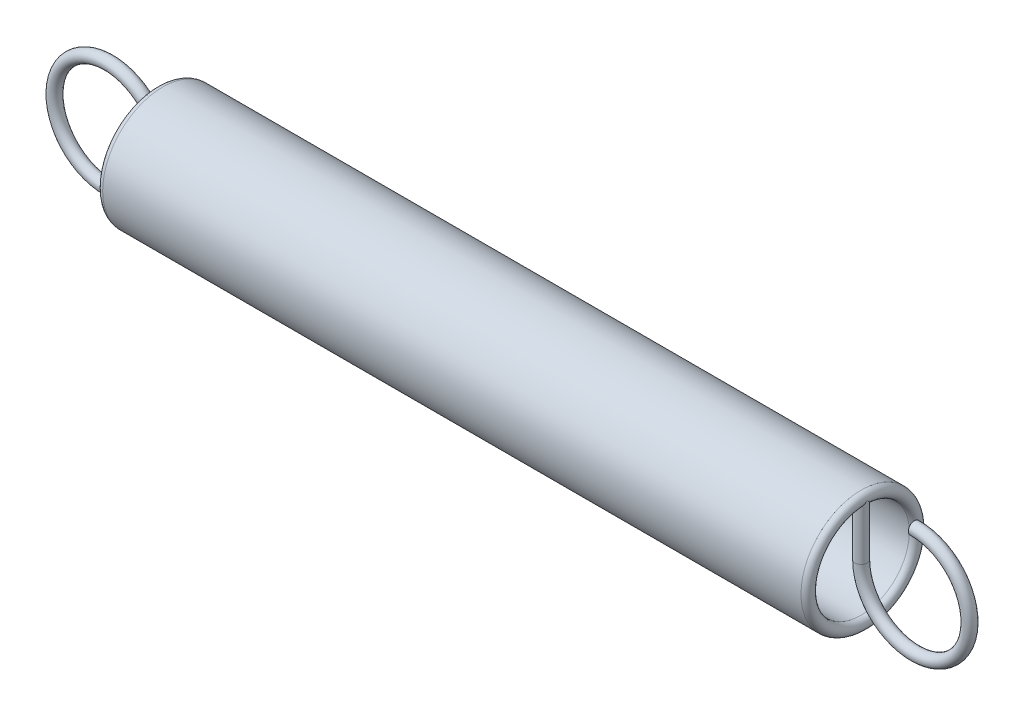
from build123d import *

# Parameters (mm, degrees)
SKETCH2_W      = 0.2
SKETCH2_H      = 1.8
SKETCH3_R      = 0.2
REVOLVE3_ANGLE = 271
SKETCH4_W      = 0.2
SKETCH4_H      = 1.8
SKETCH5_R      = 0.2
REVOLVE5_ANGLE = 271


with BuildPart() as part:
    # Sketch1 → Revolve1 (revolve)
    with BuildSketch(Plane.XY, mode=Mode.PRIVATE) as revolve1_sk:
        with BuildLine():
            Line((3.4, 1.6), (26.6, 1.6))
            ThreePointArc((26.6, 1.6), (26.8, 1.8), (26.6, 2))
            Line((26.6, 2), (3.4, 2))
            ThreePointArc((3.4, 2), (3.2, 1.8), (3.4, 1.6))
        make_face()
    revolve(revolve1_sk.sketch.rotate(Axis((26.8, 0, 0), (-1, 0, 0)), 270), axis=Axis((26.8, 0, 0), (-1, 0, 0)))

    # Sketch2 → Revolve2 (revolve)
    with BuildSketch(Plane.XY, mode=Mode.PRIVATE) as revolve2_sk:
        with Locations((26.7, 0.9)):
            Rectangle(SKETCH2_W, SKETCH2_H)
    revolve(revolve2_sk.sketch.rotate(Axis((26.6, 0, 0), (0, 1, 0)), 270), axis=Axis((26.6, 0, 0), (0, 1, 0)))

    # Sketch3 → Revolve3 (revolve)
    with BuildSketch(Plane(origin=(0, 0, 0), x_dir=(1, 0, 0), z_dir=(0, 1, 0))):
        with Locations(Location((26.6, 0, 0), (0, 0, 269.999999932))):
            Circle(SKETCH3_R)
    revolve(axis=Axis((28.4, 0, -2), (0, 0, 1)), revolution_arc=REVOLVE3_ANGLE)

    # Sketch4 → Revolve4 (revolve)
    with BuildSketch(Plane.XY, mode=Mode.PRIVATE) as revolve4_sk:
        with Locations((3.5, -0.9)):
            Rectangle(SKETCH4_W, SKETCH4_H)
    revolve(revolve4_sk.sketch.rotate(Axis((3.4, -1.8, 0), (0, 1, 0)), 90), axis=Axis((3.4, -1.8, 0), (0, 1, 0)))

    # Sketch5 → Revolve5 (revolve)
    with BuildSketch(Plane(origin=(0, 0, 0), x_dir=(1, 0, 0), z_dir=(0, 1, 0))):
        with Locations(Location((3.4, 0, 0), (0, 0, 90))):
            Circle(SKETCH5_R)
    revolve(axis=Axis((1.6, 0, 2), (0, 0, 1)), revolution_arc=REVOLVE5_ANGLE)


solid = part.part
